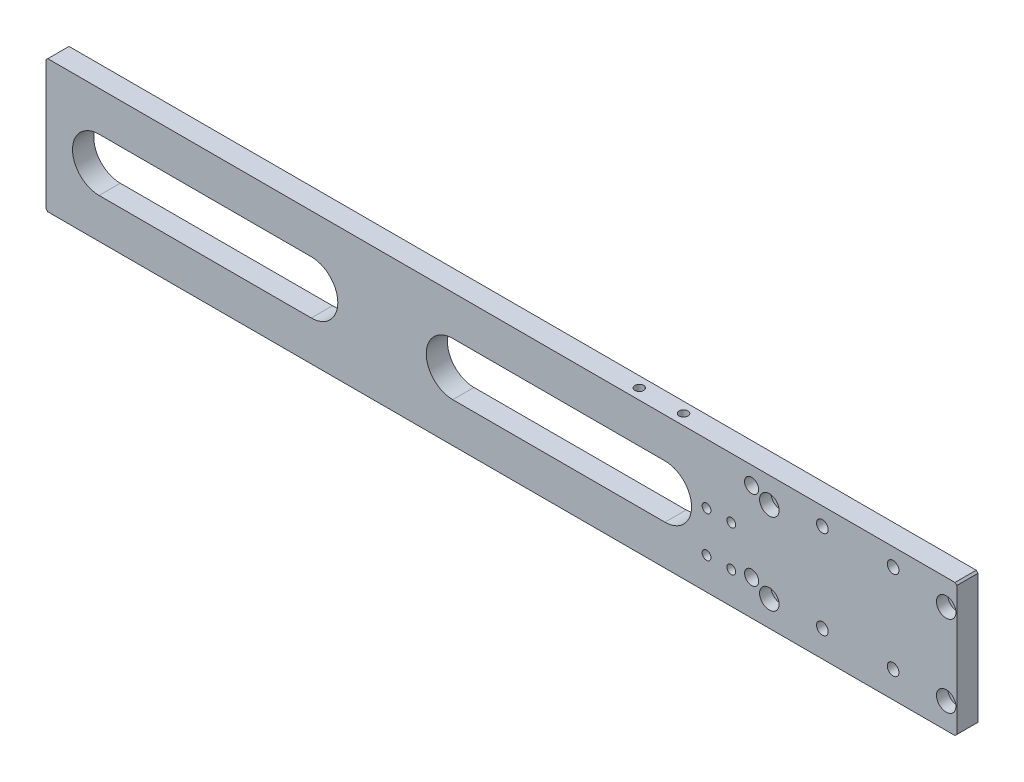
from build123d import *

# Parameters (mm, degrees)
SKETCH1_W                                           = 515
SKETCH1_H                                           = 75
BOSS_EXTRUDE1_DEPTH                                 = 6
M6_TAPPED_HOLE1_D                                   = 5
M6_TAPPED_HOLE1_DEPTH                               = 17
BLIND_PIN_HOLE2_D                                   = 8
CBORE_FOR_M6_HEX_SOCKET_HEAD_CAP_SCREW1_D           = 6.2
CBORE_FOR_M6_HEX_SOCKET_HEAD_CAP_SCREW1_CBORE_D     = 11
CBORE_FOR_M6_HEX_SOCKET_HEAD_CAP_SCREW1_CBORE_DEPTH = 6.4
M6_TAPPED_HOLE2_D                                   = 5
M6_TAPPED_HOLE3_D                                   = 5
M6_TAPPED_HOLE3_DEPTH                               = 12
M6_TAPPED_HOLE3_TIP                                 = 1.502151548
MM_2_D                                              = 5
MM_2_DEPTH                                          = 11
MM_2_TIP                                            = 1.502151548
CBORE_FOR_M6_HEX_SOCKET_HEAD_CAP_SCREW2_D           = 6.6
CBORE_FOR_M6_HEX_SOCKET_HEAD_CAP_SCREW2_CBORE_D     = 11
CBORE_FOR_M6_HEX_SOCKET_HEAD_CAP_SCREW2_CBORE_DEPTH = 6.4
CUT_EXTRUDE1_DEPTH                                  = 261.492802204
CHAMFER1_SIZE                                       = 1


with BuildPart() as part:
    # Sketch1 → Boss-Extrude1 (new, symmetric)
    with BuildSketch(Plane.XY):
        Rectangle(SKETCH1_W, SKETCH1_H)
    extrude(amount=BOSS_EXTRUDE1_DEPTH, both=True)

    # M6 Tapped Hole1
    with Locations(Plane(origin=(0, 37.5, 0), x_dir=(1, 0, 0), z_dir=(0, 1, 0))):
        with Locations((72, 0), (97, 0)):
            Hole(M6_TAPPED_HOLE1_D / 2, depth=M6_TAPPED_HOLE1_DEPTH)

    # Blind pin hole2 (through all)
    with Locations(Plane(origin=(0, 0, -6), x_dir=(-1, 0, 0), z_dir=(0, 0, -1))):
        with Locations((-141.5, 27.5), (-141.5, -17.5)):
            Hole(BLIND_PIN_HOLE2_D / 2)

    # CBORE for M6 Hex Socket Head Cap Screw1 (through all)
    with Locations(Plane.XY.offset(6)):
        with Locations((151.5, 23), (151.5, -23), (251.5, 23), (251.5, -23)):
            CounterBoreHole(CBORE_FOR_M6_HEX_SOCKET_HEAD_CAP_SCREW1_D / 2, CBORE_FOR_M6_HEX_SOCKET_HEAD_CAP_SCREW1_CBORE_D / 2, CBORE_FOR_M6_HEX_SOCKET_HEAD_CAP_SCREW1_CBORE_DEPTH)

    # M6 Tapped Hole2 (through all)
    with Locations(Plane.XY.offset(6)):
        with Locations((116.0005, 3.6), (130.0005, 3.6), (116.0005, -19.4), (130.0005, -19.4)):
            Hole(M6_TAPPED_HOLE2_D / 2)

    # M6 Tapped Hole3
    with Locations(Plane(origin=(0, -37.5, 0), x_dir=(-1, 0, 0), z_dir=(0, -1, 0))):
        with Locations((237.5, 0), (142.5, 0), (47.5, 0), (-47.5, 0), (-142.5, 0), (-237.5, 0)):
            Hole(M6_TAPPED_HOLE3_D / 2, depth=M6_TAPPED_HOLE3_DEPTH)
            with Locations((0, 0, -(M6_TAPPED_HOLE3_DEPTH + M6_TAPPED_HOLE3_TIP / 2))):  # 118° drill point
                Cone(0, M6_TAPPED_HOLE3_D / 2, M6_TAPPED_HOLE3_TIP, mode=Mode.SUBTRACT)

    # 大小mm 暗销孔2
    with Locations(Plane(origin=(0, -37.5, 0), x_dir=(-1, 0, 0), z_dir=(0, -1, 0))):
        with Locations((-197.5, 0), (197.5, 0)):
            Hole(MM_2_D / 2, depth=MM_2_DEPTH)
            with Locations((0, 0, -(MM_2_DEPTH + MM_2_TIP / 2))):  # 118° drill point
                Cone(0, MM_2_D / 2, MM_2_TIP, mode=Mode.SUBTRACT)

    # CBORE for M6 Hex Socket Head Cap Screw2 (through all)
    with Locations(Plane(origin=(0, 0, -6), x_dir=(-1, 0, 0), z_dir=(0, 0, -1))):
        with Locations((-221.5, 27.5), (-181.5, 27.5), (-181.5, -22.5), (-221.5, -22.5)):
            CounterBoreHole(CBORE_FOR_M6_HEX_SOCKET_HEAD_CAP_SCREW2_D / 2, CBORE_FOR_M6_HEX_SOCKET_HEAD_CAP_SCREW2_CBORE_D / 2, CBORE_FOR_M6_HEX_SOCKET_HEAD_CAP_SCREW2_CBORE_DEPTH)

    # Sketch18 → Cut-Extrude1 (cut, through all)
    with BuildSketch(Plane.XY.offset(6)):
        with BuildLine():
            Line((-227.5, 15), (-107.5, 15))
            ThreePointArc((-107.5, 15), (-92.5, 0), (-107.5, -15))
            Line((-107.5, -15), (-227.5, -15))
            ThreePointArc((-227.5, -15), (-242.5, 0), (-227.5, 15))
        make_face()
        with BuildLine():
            Line((-27.5, 15), (92.5, 15))
            ThreePointArc((92.5, 15), (107.5, 0), (92.5, -15))
            Line((92.5, -15), (-27.5, -15))
            ThreePointArc((-27.5, -15), (-42.5, 0), (-27.5, 15))
        make_face()
    extrude(amount=-CUT_EXTRUDE1_DEPTH, mode=Mode.SUBTRACT)

    # Chamfer1
    chamfer1_edges = [part.edges().sort_by_distance(p)[0] for p in [
        (257.5, -37.5, 0),
        (-257.5, -37.5, 0),
        (-257.5, 37.5, 0),
        (257.5, 37.5, 0),
    ]]
    chamfer(chamfer1_edges, length=CHAMFER1_SIZE)


solid = part.part
